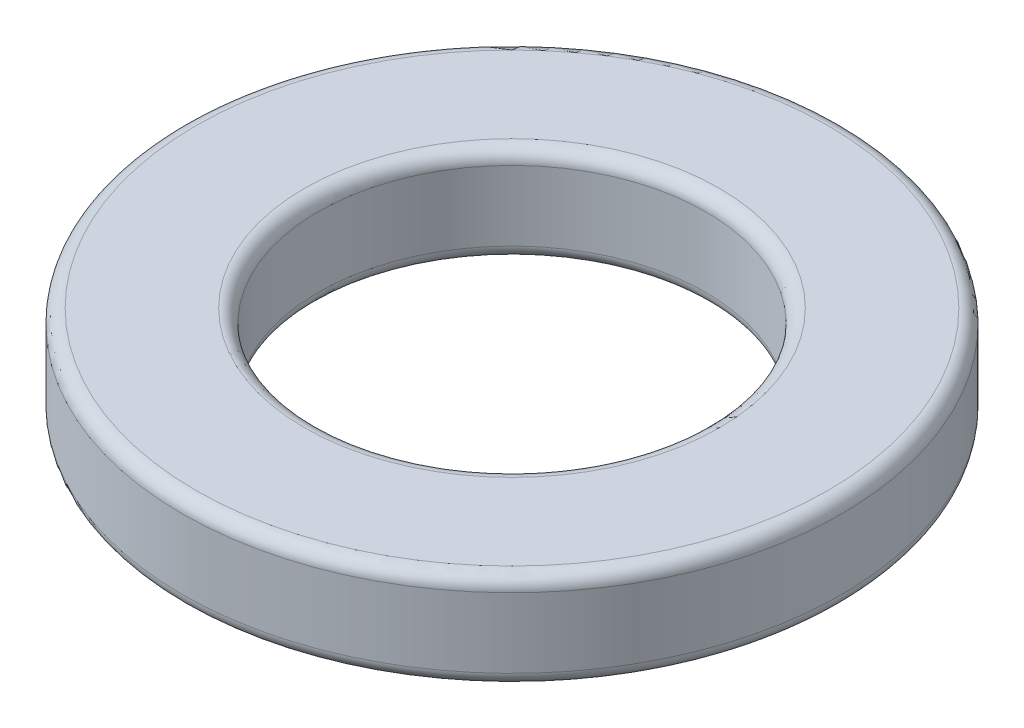
SolidWorks part; units mm, degrees
material "AISI 304"
ref_plane "前视基准面" through (0, 0, 0) normal (0, 0, 1) x (1, 0, 0)
ref_plane "上视基准面" through (0, 0, 0) normal (0, 1, 0) x (1, 0, 0)
ref_plane "右视基准面" through (0, 0, 0) normal (1, 0, 0) x (0, 0, -1)
sketch "草图1" plane through (0, 0, 0) normal (0, 1, 0) x (1, 0, 0)
  circle A0 centre (0, 0) radius 1.7
  circle A1 centre (0, 0) radius 1
  dimension "D1" = 2
  dimension "D2" = 0.7
extrude "凸台-拉伸1" add sketch "草图1" along normal blind 0.5
fillet "圆角1" radius 0.07 4 edges at (0, 0, 1) (0, 0.5, 1) (0, 0, 1.7) (0, 0.5, 1.7)
